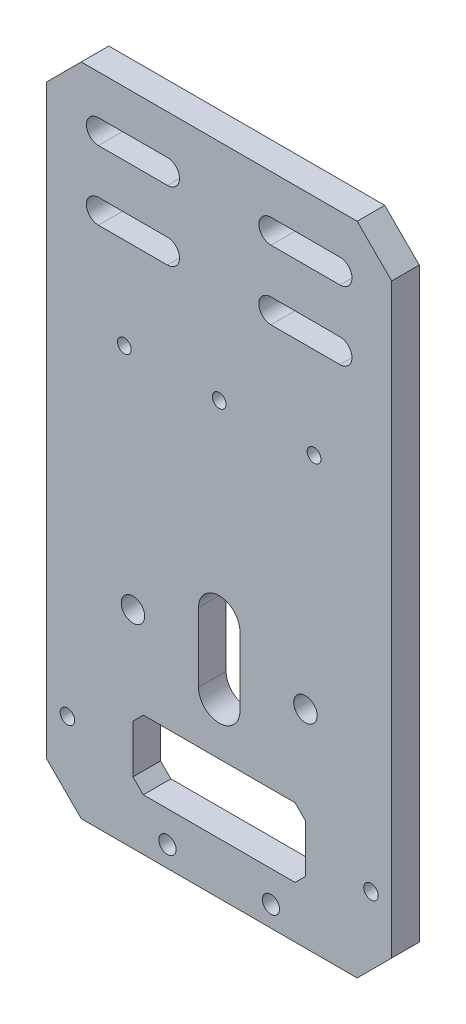
from build123d import *

# Parameters (mm, degrees)
SKETCH1_R                   = 2.5
SKETCH1_R_2                 = 2
SKETCH1_W                   = 50
SKETCH1_H                   = 20
BOSS_EXTRUDE1_DEPTH         = 8
CHAMFER1_SIZE               = 3
TAP_DRILL_FOR_M8_TAP1_D     = 6.8
TAP_DRILL_FOR_M8_TAP1_DEPTH = 15
TAP_DRILL_FOR_M8_TAP1_TIP   = 2.042926105
TAP_DRILL_FOR_M5_TAP1_D     = 4.2
TAP_DRILL_FOR_M5_TAP1_DEPTH = 15
TAP_DRILL_FOR_M5_TAP1_TIP   = 1.2618073
CUT_EXTRUDE1_DEPTH          = 10
LPATTERN1_COUNT             = 2
LPATTERN1_PITCH             = 20


with BuildPart() as part:
    # Sketch1 → Boss-Extrude1 (new body)
    with BuildSketch(Plane.XY):
        Polygon((0, 180), (10, 190), (90, 190), (100, 180), (100, 10), (90, 0), (10, 0), (0, 10), align=None)
        with Locations((35, 6)):
            Circle(SKETCH1_R, mode=Mode.SUBTRACT)
        with Locations((65, 6)):
            Circle(SKETCH1_R, mode=Mode.SUBTRACT)
        with Locations((22.5, 125)):
            Circle(SKETCH1_R_2, mode=Mode.SUBTRACT)
        with Locations((50, 125)):
            Circle(SKETCH1_R_2, mode=Mode.SUBTRACT)
        with Locations((77.5, 125)):
            Circle(SKETCH1_R_2, mode=Mode.SUBTRACT)
        with Locations((50, 25)):
            Rectangle(SKETCH1_W, SKETCH1_H, mode=Mode.SUBTRACT)
        with BuildLine():
            Line((56, 70), (56, 50))
            ThreePointArc((56, 50), (50, 44), (44, 50))
            Line((44, 50), (44, 70))
            ThreePointArc((44, 70), (50, 76), (56, 70))
        make_face(mode=Mode.SUBTRACT)
    extrude(amount=BOSS_EXTRUDE1_DEPTH)

    # Chamfer1
    chamfer1_edges = [part.edges().sort_by_distance(p)[0] for p in [
        (25, 35, 4),
        (25, 15, 4),
        (75, 15, 4),
        (75, 35, 4),
    ]]
    chamfer(chamfer1_edges, length=CHAMFER1_SIZE)

    # Tap Drill for M8 Tap1
    with Locations(Plane(origin=(25, 60, 8), x_dir=(1, 0, 0), z_dir=(0, 0, 1))):
        with Locations((0, 0), (50, 0)):
            Hole(TAP_DRILL_FOR_M8_TAP1_D / 2, depth=TAP_DRILL_FOR_M8_TAP1_DEPTH)
            with Locations((0, 0, -(TAP_DRILL_FOR_M8_TAP1_DEPTH + TAP_DRILL_FOR_M8_TAP1_TIP / 2))):  # 118° drill point
                Cone(0, TAP_DRILL_FOR_M8_TAP1_D / 2, TAP_DRILL_FOR_M8_TAP1_TIP, mode=Mode.SUBTRACT)

    # Tap Drill for M5 Tap1
    with Locations(Plane(origin=(94, 23.685438565, 0), x_dir=(-1, 0, 0), z_dir=(0, 0, -1))):
        with Locations((0, 0), (88, 0)):
            Hole(TAP_DRILL_FOR_M5_TAP1_D / 2, depth=TAP_DRILL_FOR_M5_TAP1_DEPTH)
            with Locations((0, 0, -(TAP_DRILL_FOR_M5_TAP1_DEPTH + TAP_DRILL_FOR_M5_TAP1_TIP / 2))):  # 118° drill point
                Cone(0, TAP_DRILL_FOR_M5_TAP1_D / 2, TAP_DRILL_FOR_M5_TAP1_TIP, mode=Mode.SUBTRACT)

    # Sketch5 → Cut-Extrude1 (cut)
    with BuildSketch(Plane(origin=(0, 0, 0), x_dir=(-1, 0, 0), z_dir=(0, 0, -1))):
        with BuildLine():
            Line((-85, 178.5), (-65, 178.5))
            ThreePointArc((-65, 178.5), (-61.5, 175), (-65, 171.5))
            Line((-65, 171.5), (-85, 171.5))
            ThreePointArc((-85, 171.5), (-88.5, 175), (-85, 178.5))
        make_face()
        with BuildLine():
            Line((-15, 178.5), (-35, 178.5))
            ThreePointArc((-35, 178.5), (-38.5, 175), (-35, 171.5))
            Line((-35, 171.5), (-15, 171.5))
            ThreePointArc((-15, 171.5), (-11.5, 175), (-15, 178.5))
        make_face()
    cut_extrude1 = extrude(amount=-CUT_EXTRUDE1_DEPTH, mode=Mode.SUBTRACT)

    # LPattern1: Cut-Extrude1 ×2
    with Locations(*[(0, -i * LPATTERN1_PITCH, 0) for i in range(1, LPATTERN1_COUNT)]):
        add(cut_extrude1, mode=Mode.SUBTRACT)


solid = part.part
